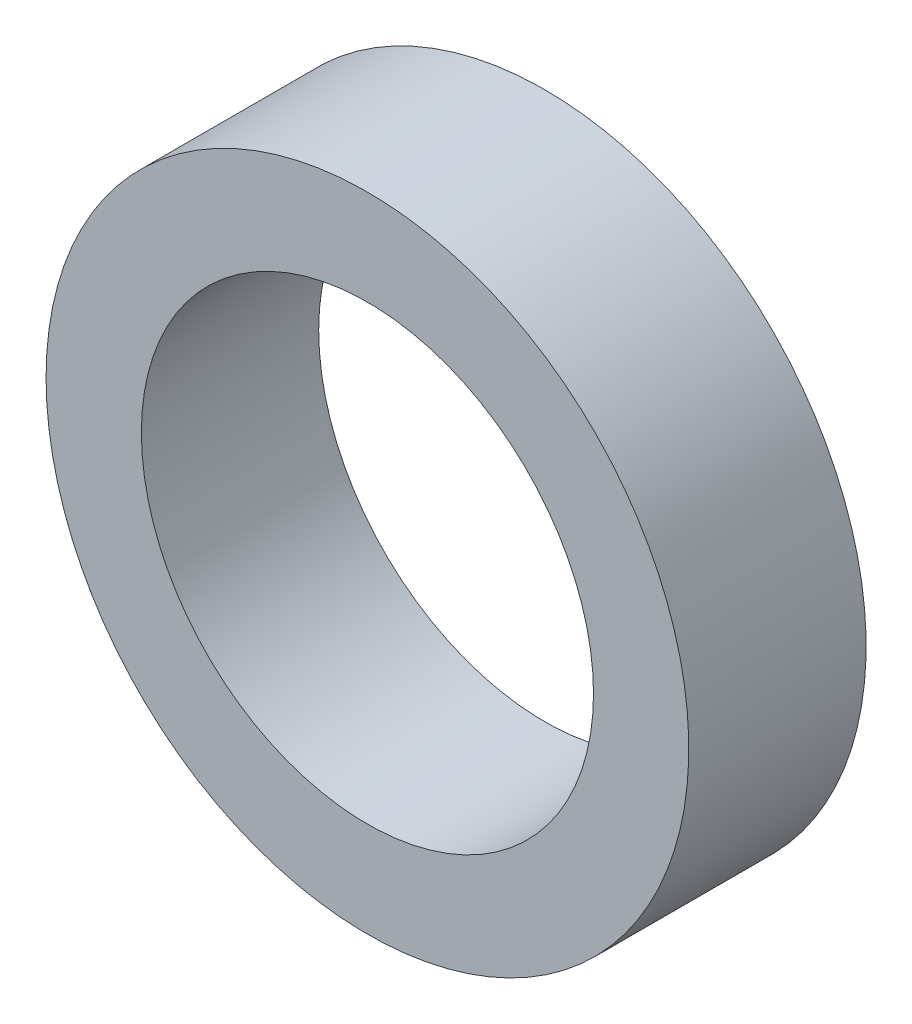
SolidWorks part; units mm, degrees
material "1023 碳钢板 (SS)"
ref_plane "Front Plane" through (0, 0, 0) normal (0, 0, 1) x (1, 0, 0)
ref_plane "Top Plane" through (0, 0, 0) normal (0, 1, 0) x (1, 0, 0)
ref_plane "Right Plane" through (0, 0, 0) normal (1, 0, 0) x (0, 0, -1)
ref_plane "Plane4" through (0, 0, 0) normal (0, -1, 0) x (1, 0, 0)
sketch "Sketch1" plane through (0, 0, 0) normal (0, -1, 0) x (1, 0, 0)
  line L0 (5.1, -2) -> (7.25, -2)
  line L1 (7.25, -2) -> (7.25, 2)
  line L2 (7.25, 2) -> (5.1, 2)
  line L3 (5.1, 2) -> (5.1, -2)
  line L4 (0, 2) -> (0, -2) construction
revolve "Revolve1" add sketch "Sketch1" angle 360 about L4
